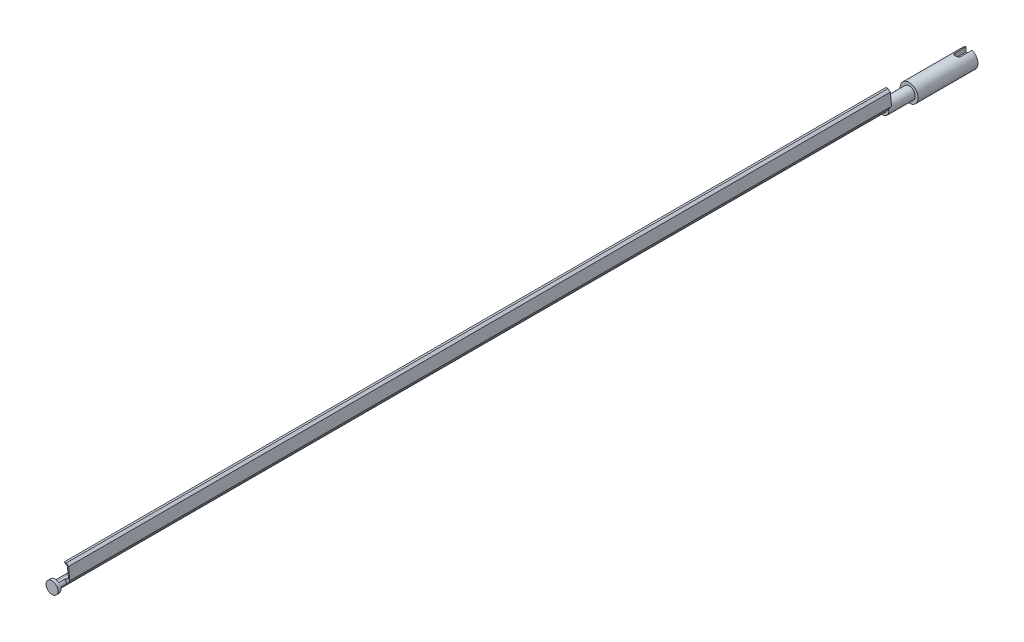
from build123d import *

# Parameters (mm, degrees)
SKETCH1_R           = 100
BOSS_EXTRUDE1_DEPTH = 50
BOSS_EXTRUDE2_DEPTH = 13824
BOSS_EXTRUDE3_START = 440
SKETCH3_R           = 100
BOSS_EXTRUDE3_DEPTH = 440
CUT_EXTRUDE1_START  = -100
CUT_EXTRUDE1_DEPTH  = 100
SKETCH6_R           = 150
BOSS_EXTRUDE5_DEPTH = 2000
CUT_EXTRUDE2_DEPTH  = 326
BOSS_EXTRUDE6_DEPTH = 75
BOSS_EXTRUDE7_START = 1000
SKETCH9_R           = 150
BOSS_EXTRUDE7_DEPTH = 1000
CUT_EXTRUDE3_START  = 65
CUT_EXTRUDE3_DEPTH  = 300
SKETCH11_W          = 300
SKETCH11_H          = 2000
CUT_EXTRUDE4_DEPTH  = 250


with BuildPart() as part:
    # Sketch1 → Boss-Extrude1 (new body)
    with BuildSketch(Plane.XY):
        Circle(SKETCH1_R)
    extrude(amount=BOSS_EXTRUDE1_DEPTH)

    # Sketch2 → Boss-Extrude2 (add)
    with BuildSketch(Plane(origin=(0, 0, 0), x_dir=(-1, 0, 0), z_dir=(0, 0, -1))):
        with BuildLine():
            Line((-96.233395069, 27.187012957), (-146.428749083, 97.201990132))
            Line((-146.428749083, 97.201990132), (-127.238656611, 294.943377783))
            Line((-127.238656611, 294.943377783), (-85.855376139, 324.612007229))
            Line((-85.855376139, 324.612007229), (-53.815694107, 324.612007229))
            Line((-53.815694107, 324.612007229), (-69.835535123, 313.127013254))
            Line((-69.835535123, 313.127013254), (-106.547016375, 286.807704556))
            Line((-106.547016375, 286.807704556), (-127.238656611, 110.959810588))
            Line((-127.238656611, 110.959810588), (-61.825614615, 78.597667761))
            Line((-61.825614615, 78.597667761), (0, 58.675035722))
            ThreePointArc((0, 58.675035722), (51.995426196, -27.188885075), (-48.18736452, -33.477421012))
            Line((-48.18736452, -33.477421012), (-96.233395069, 27.187012957))
        make_face()
    extrude(amount=BOSS_EXTRUDE2_DEPTH)

    # Sketch3 → Boss-Extrude3 (add)
    with BuildSketch(Plane(origin=(0, 0, -13824), x_dir=(-1, 0, 0), z_dir=(0, 0, -1)).offset(BOSS_EXTRUDE3_START)):
        with Locations(Location((0, 0, 0), (0, 0, 128.188900559))):
            Circle(SKETCH3_R)
    extrude(amount=-BOSS_EXTRUDE3_DEPTH)

    # Sketch4 → Cut-Extrude1 (cut)
    with BuildSketch(Plane.XY.offset(CUT_EXTRUDE1_START)):
        with BuildLine():
            Line((96.233395069, 27.187012957), (146.428749083, 97.201990132))
            Line((146.428749083, 97.201990132), (127.238656611, 294.943377783))
            Line((127.238656611, 294.943377783), (85.855376139, 324.612007229))
            Line((85.855376139, 324.612007229), (53.815694107, 324.612007229))
            Line((53.815694107, 324.612007229), (106.547016375, 286.807704556))
            Line((106.547016375, 286.807704556), (127.238656611, 110.959810588))
            Line((127.238656611, 110.959810588), (61.825614615, 78.597667761))
            ThreePointArc((61.825614615, 78.597667761), (83.104912565, 55.619902082), (96.233395069, 27.187012957))
        make_face()
    extrude(amount=CUT_EXTRUDE1_DEPTH, mode=Mode.SUBTRACT)

    # Sketch6 → Boss-Extrude5 (add)
    with BuildSketch(Plane.XY.offset(50)):
        Circle(SKETCH6_R)
    extrude(amount=BOSS_EXTRUDE5_DEPTH)

    # Sketch7 → Cut-Extrude2 (cut)
    with BuildSketch(Plane(origin=(0, 0, 0), x_dir=(1, 0, 0), z_dir=(0, 1, 0))):
        with BuildLine():
            Line((50, -1600), (50, -1900))
            ThreePointArc((50, -1900), (0, -1950), (-50, -1900))
            Line((-50, -1900), (-50, -1600))
            ThreePointArc((-50, -1600), (0, -1550), (50, -1600))
        make_face()
    extrude(amount=CUT_EXTRUDE2_DEPTH, mode=Mode.SUBTRACT)

    # Sketch8 → Boss-Extrude6 (add)
    with BuildSketch(Plane(origin=(0, 0, 0), x_dir=(1, 0, 0), z_dir=(0, 1, 0))):
        with BuildLine():
            Line((-50, -1600), (-50, -1900))
            ThreePointArc((-50, -1900), (0, -1950), (50, -1900))
            Line((50, -1900), (50, -1600))
            ThreePointArc((50, -1600), (0, -1550), (-50, -1600))
        make_face()
    extrude(amount=BOSS_EXTRUDE6_DEPTH)

    # Sketch9 → Boss-Extrude7 (add)
    with BuildSketch(Plane(origin=(0, 0, -14264), x_dir=(-1, 0, 0), z_dir=(0, 0, -1)).offset(BOSS_EXTRUDE7_START)):
        with Locations(Location((0, 0, 0), (0, 0, 180))):
            Circle(SKETCH9_R)
    extrude(amount=-BOSS_EXTRUDE7_DEPTH)

    # Sketch10 → Cut-Extrude3 (cut)
    with BuildSketch(Plane(origin=(0, 0, 0), x_dir=(1, 0, 0), z_dir=(0, 1, 0)).offset(CUT_EXTRUDE3_START)):
        with BuildLine():
            Line((50, 15384), (50, 15084))
            ThreePointArc((50, 15084), (0, 15034), (-50, 15084))
            Line((-50, 15084), (-50, 15384))
            ThreePointArc((-50, 15384), (0, 15434), (50, 15384))
        make_face()
    extrude(amount=CUT_EXTRUDE3_DEPTH, mode=Mode.SUBTRACT)

    # Sketch11 → Cut-Extrude4 (cut, symmetric)
    with BuildSketch(Plane(origin=(0, 0, 0), x_dir=(1, 0, 0), z_dir=(0, 1, 0))):
        with Locations((0, -1050)):
            Rectangle(SKETCH11_W, SKETCH11_H)
    extrude(amount=CUT_EXTRUDE4_DEPTH, both=True, mode=Mode.SUBTRACT)


solid = part.part
